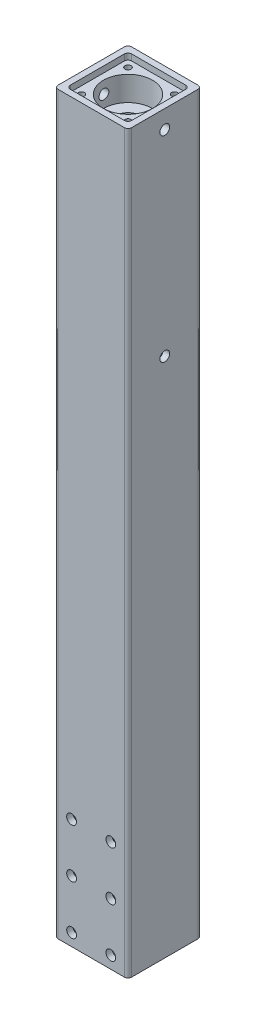
from build123d import *

# Parameters (mm, degrees)
SKETCH1_W               = 60
SKETCH1_H               = 60
BOSS_EXTRUDE1_DEPTH     = 600
SKETCH2_W               = 50
SKETCH2_H               = 50
CUT_EXTRUDE1_DEPTH      = 5
CUT_EXTRUDE3_DEPTH      = 600
CUT_EXTRUDE3_DEPTH_BACK = 30
SKETCH4_R               = 4
FILLET2_R               = 3
SKETCH3_R               = 20
CUT_EXTRUDE4_DEPTH      = 20
SKETCH5_W               = 50
SKETCH5_H               = 50
CUT_EXTRUDE5_DEPTH      = 110
SKETCH6_R               = 25
CUT_EXTRUDE6_DEPTH      = 450
SKETCH7_R               = 10
CUT_EXTRUDE7_DEPTH      = 15
FILLET4_R               = 3
CUT_EXTRUDE8_DEPTH      = 30
CUT_EXTRUDE8_DEPTH_BACK = 30
SKETCH8_R               = 4
CUT_EXTRUDE9_DEPTH      = 30
CUT_EXTRUDE9_DEPTH_BACK = 30
SKETCH9_R               = 4
SKETCH10_R              = 2.5
CUT_EXTRUDE10_DEPTH     = 20


with BuildPart() as part:
    # Sketch1 → Boss-Extrude1 (new body)
    with BuildSketch(Plane(origin=(0, 0, 0), x_dir=(1, 0, 0), z_dir=(0, 1, 0))):
        Rectangle(SKETCH1_W, SKETCH1_H)
    extrude(amount=BOSS_EXTRUDE1_DEPTH)

    # Sketch2 → Cut-Extrude1 (cut)
    with BuildSketch(Plane(origin=(0, 600, 0), x_dir=(1, 0, 0), z_dir=(0, 1, 0))):
        Rectangle(SKETCH2_W, SKETCH2_H)
    extrude(amount=-CUT_EXTRUDE1_DEPTH, mode=Mode.SUBTRACT)

    # Sketch4 → Cut-Extrude3 (cut, two sides: drawn at the far end of the back side and taken through both)
    with BuildSketch(Plane(origin=(0, 0, 0), x_dir=(0, 0, -1), z_dir=(1, 0, 0)).offset(-CUT_EXTRUDE3_DEPTH_BACK)):
        with Locations(Location((0, 585, 0), (0, 0, 180))):
            Circle(SKETCH4_R)
    extrude(amount=CUT_EXTRUDE3_DEPTH + CUT_EXTRUDE3_DEPTH_BACK, mode=Mode.SUBTRACT)

    # Fillet2
    fillet2_edges = [part.edges().sort_by_distance(p)[0] for p in [
        (30, 300, 30),
        (-30, 300, 30),
        (-30, 300, -30),
        (30, 300, -30),
    ]]
    fillet(fillet2_edges, radius=FILLET2_R)

    # Sketch3 → Cut-Extrude4 (cut)
    with BuildSketch(Plane(origin=(0, 595, 0), x_dir=(1, 0, 0), z_dir=(0, 1, 0))):
        with Locations(Location((0, 0, 0), (0, 0, 270))):
            Circle(SKETCH3_R)
    extrude(amount=-CUT_EXTRUDE4_DEPTH, mode=Mode.SUBTRACT)

    # Sketch5 → Cut-Extrude5 (cut)
    with BuildSketch(Plane.XZ):
        Rectangle(SKETCH5_W, SKETCH5_H)
    extrude(amount=-CUT_EXTRUDE5_DEPTH, mode=Mode.SUBTRACT)

    # Sketch6 → Cut-Extrude6 (cut)
    with BuildSketch(Plane.XZ.offset(-110)):
        with Locations(Location((0, 0, 0), (0, 0, 270))):
            Circle(SKETCH6_R)
    extrude(amount=-CUT_EXTRUDE6_DEPTH, mode=Mode.SUBTRACT)

    # Sketch7 → Cut-Extrude7 (cut)
    with BuildSketch(Plane(origin=(0, 575, 0), x_dir=(1, 0, 0), z_dir=(0, 1, 0))):
        with Locations(Location((0, 0, 0), (0, 0, 270))):
            Circle(SKETCH7_R)
    extrude(amount=-CUT_EXTRUDE7_DEPTH, mode=Mode.SUBTRACT)

    # Fillet4
    fillet4_edges = [part.edges().sort_by_distance(p)[0] for p in [
        (25, 597.5, -25),
        (25, 597.5, 25),
        (-25, 597.5, 25),
        (-25, 597.5, -25),
    ]]
    fillet(fillet4_edges, radius=FILLET4_R)

    # Sketch8 → Cut-Extrude8 (cut, two sides: drawn at the far end of the back side and taken through both)
    with BuildSketch(Plane(origin=(0, 0, 0), x_dir=(0, 0, -1), z_dir=(1, 0, 0)).offset(-CUT_EXTRUDE8_DEPTH_BACK)):
        with Locations(Location((0, 425, 0), (0, 0, 180))):
            Circle(SKETCH8_R)
    extrude(amount=CUT_EXTRUDE8_DEPTH + CUT_EXTRUDE8_DEPTH_BACK, mode=Mode.SUBTRACT)

    # Sketch9 → Cut-Extrude9 (cut, two sides: drawn at the far end of the back side and taken through both)
    with BuildSketch(Plane.XY.offset(-CUT_EXTRUDE9_DEPTH_BACK)):
        with Locations((-16, 50)):
            Circle(SKETCH9_R)
        with Locations((16, 90)):
            Circle(SKETCH9_R)
        with Locations((16, 50)):
            Circle(SKETCH9_R)
        with Locations((-16, 90)):
            Circle(SKETCH9_R)
        with Locations(Location((16, 10, 0), (0, 0, 180))):
            Circle(SKETCH9_R)
        with Locations((-16, 10)):
            Circle(SKETCH9_R)
    extrude(amount=CUT_EXTRUDE9_DEPTH + CUT_EXTRUDE9_DEPTH_BACK, mode=Mode.SUBTRACT)

    # Sketch10 → Cut-Extrude10 (cut)
    with BuildSketch(Plane(origin=(0, 595, 0), x_dir=(1, 0, 0), z_dir=(0, 1, 0))):
        with Locations(Location((-19, 19, 0), (0, 0, 270))):
            Circle(SKETCH10_R)
        with Locations(Location((19, 19, 0), (0, 0, 270))):
            Circle(SKETCH10_R)
        with Locations(Location((19, -19, 0), (0, 0, 270))):
            Circle(SKETCH10_R)
        with Locations(Location((-19, -19, 0), (0, 0, 270))):
            Circle(SKETCH10_R)
    extrude(amount=-CUT_EXTRUDE10_DEPTH, mode=Mode.SUBTRACT)


solid = part.part
